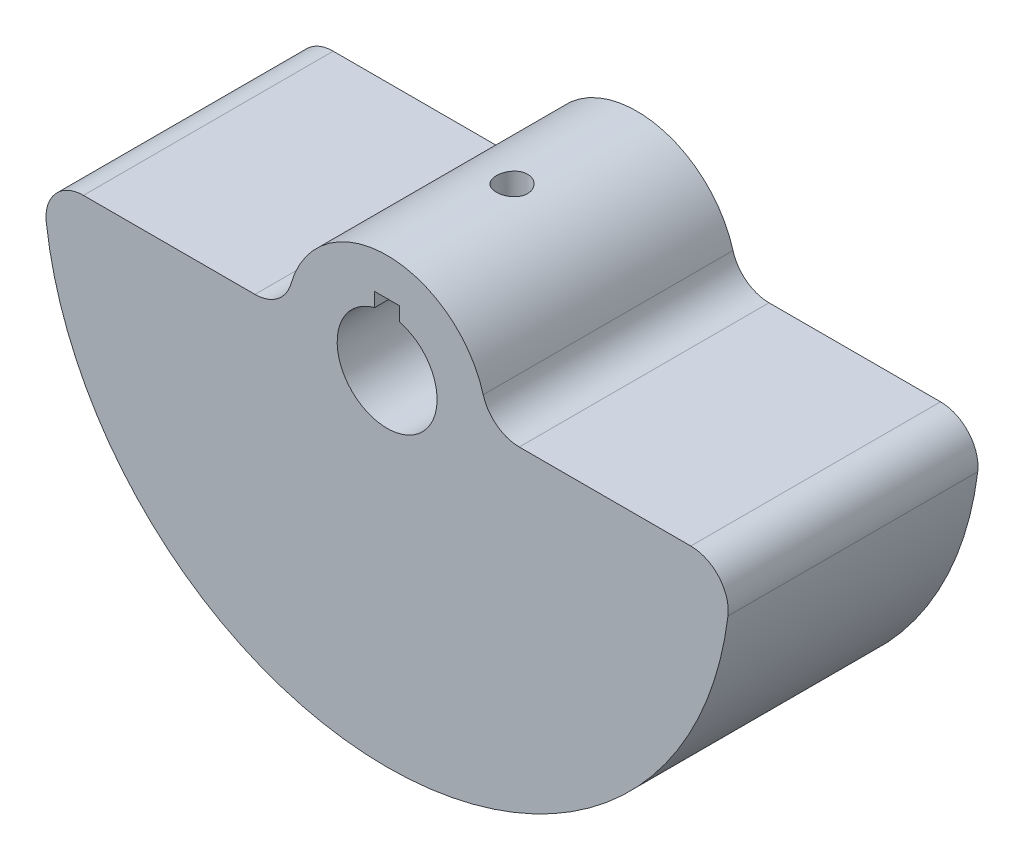
SolidWorks part; units mm, degrees
material "Q235A"
ref_plane "前视基准面" through (0, 0, 0) normal (0, 0, 1) x (1, 0, 0)
ref_plane "上视基准面" through (0, 0, 0) normal (0, 1, 0) x (1, 0, 0)
ref_plane "右视基准面" through (0, 0, 0) normal (1, 0, 0) x (0, 0, -1)
sketch "草图2" plane through (0, 0, 0) normal (0, 0, 1) x (1, 0, 0)
  line L0 (-27.5, 0) -> (27.5, 0)
  arc A0 (-27.5, 0) -> (27.5, 0) centre (0, 0) ccw
  dimension "D1" = 55
extrude "凸台-拉伸1" add sketch "草图2" along normal blind 20
sketch "草图3" plane through (0, 0, 20) normal (0, 0, 1) x (1, 0, 0)
  circle A0 centre (0, 0) radius 8
  dimension "D1" = 16
extrude "凸台-拉伸2" add sketch "草图3" against normal through all
sketch "草图4" plane through (0, 0, 20) normal (0, 0, 1) x (1, 0, 0)
  circle A0 centre (0, 0) radius 4
  dimension "D1" = 8
extrude "切除-拉伸1" cut sketch "草图4" against normal through all
fillet "圆角1" radius 3 4 edges at (27.5, 0, 10) (-27.5, 0, 10) (8, 0, 10) (-8, 0, 10)
sketch "草图5" plane through (0, 0, 20) normal (0, 0, 1) x (1, 0, 0)
  line L1 (-1, 3) -> (1, 3)
  line L2 (-1, 3) -> (-1, 5)
  line L3 (-1, 5) -> (1, 5)
  line L4 (1, 3) -> (1, 5)
  line L5 (-1, 3) -> (1, 5) construction
  line L6 (-1, 5) -> (1, 3) construction
  circle A0 centre (0, 0) radius 4 construction
  point P0 (0, 4)
  dimension "D1" = 2
  dimension "D2" = 1
extrude "切除-拉伸2" cut sketch "草图5" against normal through all
ref_plane "基准面1" through (0, 8, 0) normal (0, 1, 0) x (1, 0, 0)
hole_wizard "M3 螺纹孔1" positions "草图6" profile "草图7" tap size "M3" standard "ISO"
sketch "草图6" plane through (0, 8, 0) normal (0, 1, 0) x (1, 0, 0)
  line L0 (0, 0) -> (0, -20)
  line L1 (-7.6967, -20) -> (7.6967, -20) construction
  point P0 (0, -10)
cosmetic thread "孔螺蚊线1" parameters "D1"=3.15, "D2"=3
sketch "草图7" plane through (0, 8, 10) normal (1, 0, 0) x (0, 0, 1)
  line L0 (0, 0) -> (0, 12.7511)
  line L1 (0, 12.7511) -> (1.25, 12)
  line L2 (1.25, 12) -> (1.25, 0)
  line L5 (1.25, 0) -> (0, 0)
  line L10 (0, 12.7511) -> (-1.25, 12) construction
  line L11 (0, -6.35) -> (0, 107.95) construction
  dimension "螺纹孔钻头直径" = 2.5
  dimension "螺纹孔钻头深度" = 12
  dimension "导头角度" = 118
